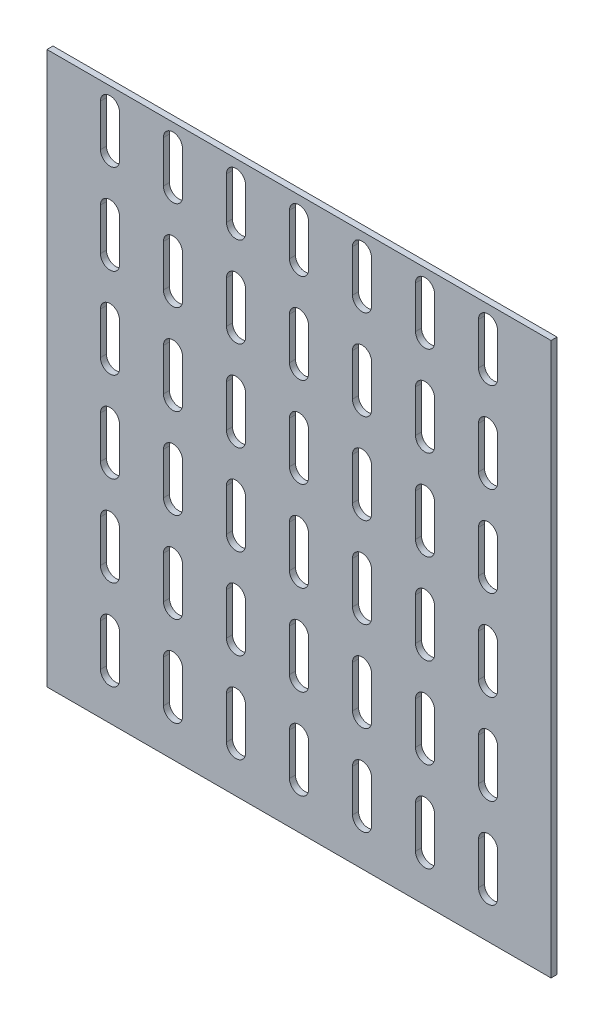
from build123d import *

# Parameters (mm, degrees)
SKETCH1_W           = 840
SKETCH1_H           = 920
BOSS_EXTRUDE1_DEPTH = 10
CUT_EXTRUDE1_DEPTH  = 10


with BuildPart() as part:
    # Sketch1 → Boss-Extrude1 (new body)
    with BuildSketch(Plane.XY):
        with Locations((368.938021937, -411.010102206)):
            Rectangle(SKETCH1_W, SKETCH1_H)
    extrude(amount=BOSS_EXTRUDE1_DEPTH)

    # Sketch2 → Cut-Extrude1 (cut)
    with BuildSketch(Plane.XY.offset(10)):
        with BuildLine():
            Line((69.818326735, -731.010102206), (69.818326735, -801.010102206))
            ThreePointArc((69.818326735, -801.010102206), (53.938021937, -816.890407004), (38.057717139, -801.010102206))
            Line((38.057717139, -801.010102206), (38.057717139, -731.010102206))
            ThreePointArc((38.057717139, -731.010102206), (53.938021937, -715.129797408), (69.818326735, -731.010102206))
        make_face()
        with BuildLine():
            Line((174.818326735, -731.010102206), (174.818326735, -801.010102206))
            ThreePointArc((174.818326735, -801.010102206), (158.938021937, -816.890407004), (143.057717139, -801.010102206))
            Line((143.057717139, -801.010102206), (143.057717139, -731.010102206))
            ThreePointArc((143.057717139, -731.010102206), (158.938021937, -715.129797408), (174.818326735, -731.010102206))
        make_face()
        with BuildLine():
            Line((69.818326735, 18.989897794), (69.818326735, -51.010102206))
            ThreePointArc((69.818326735, -51.010102206), (53.938021937, -66.890407004), (38.057717139, -51.010102206))
            Line((38.057717139, -51.010102206), (38.057717139, 18.989897794))
            ThreePointArc((38.057717139, 18.989897794), (53.938021937, 34.870202592), (69.818326735, 18.989897794))
        make_face()
        with BuildLine():
            Line((174.818326735, 18.989897794), (174.818326735, -51.010102206))
            ThreePointArc((174.818326735, -51.010102206), (158.938021937, -66.890407004), (143.057717139, -51.010102206))
            Line((143.057717139, -51.010102206), (143.057717139, 18.989897794))
            ThreePointArc((143.057717139, 18.989897794), (158.938021937, 34.870202592), (174.818326735, 18.989897794))
        make_face()
        with BuildLine():
            Line((279.818326735, 18.989897794), (279.818326735, -51.010102206))
            ThreePointArc((279.818326735, -51.010102206), (263.938021937, -66.890407004), (248.057717139, -51.010102206))
            Line((248.057717139, -51.010102206), (248.057717139, 18.989897794))
            ThreePointArc((248.057717139, 18.989897794), (263.938021937, 34.870202592), (279.818326735, 18.989897794))
        make_face()
        with BuildLine():
            Line((384.818326735, 18.989897794), (384.818326735, -51.010102206))
            ThreePointArc((384.818326735, -51.010102206), (368.938021937, -66.890407004), (353.057717139, -51.010102206))
            Line((353.057717139, -51.010102206), (353.057717139, 18.989897794))
            ThreePointArc((353.057717139, 18.989897794), (368.938021937, 34.870202592), (384.818326735, 18.989897794))
        make_face()
        with BuildLine():
            Line((489.818326735, 18.989897794), (489.818326735, -51.010102206))
            ThreePointArc((489.818326735, -51.010102206), (473.938021937, -66.890407004), (458.057717139, -51.010102206))
            Line((458.057717139, -51.010102206), (458.057717139, 18.989897794))
            ThreePointArc((458.057717139, 18.989897794), (473.938021937, 34.870202592), (489.818326735, 18.989897794))
        make_face()
        with BuildLine():
            Line((594.818326735, 18.989897794), (594.818326735, -51.010102206))
            ThreePointArc((594.818326735, -51.010102206), (578.938021937, -66.890407004), (563.057717139, -51.010102206))
            Line((563.057717139, -51.010102206), (563.057717139, 18.989897794))
            ThreePointArc((563.057717139, 18.989897794), (578.938021937, 34.870202592), (594.818326735, 18.989897794))
        make_face()
        with BuildLine():
            Line((699.818326735, 18.989897794), (699.818326735, -51.010102206))
            ThreePointArc((699.818326735, -51.010102206), (683.938021937, -66.890407004), (668.057717139, -51.010102206))
            Line((668.057717139, -51.010102206), (668.057717139, 18.989897794))
            ThreePointArc((668.057717139, 18.989897794), (683.938021937, 34.870202592), (699.818326735, 18.989897794))
        make_face()
        with BuildLine():
            Line((69.818326735, -131.010102206), (69.818326735, -201.010102206))
            ThreePointArc((69.818326735, -201.010102206), (53.938021937, -216.890407004), (38.057717139, -201.010102206))
            Line((38.057717139, -201.010102206), (38.057717139, -131.010102206))
            ThreePointArc((38.057717139, -131.010102206), (53.938021937, -115.129797408), (69.818326735, -131.010102206))
        make_face()
        with BuildLine():
            Line((174.818326735, -131.010102206), (174.818326735, -201.010102206))
            ThreePointArc((174.818326735, -201.010102206), (158.938021937, -216.890407004), (143.057717139, -201.010102206))
            Line((143.057717139, -201.010102206), (143.057717139, -131.010102206))
            ThreePointArc((143.057717139, -131.010102206), (158.938021937, -115.129797408), (174.818326735, -131.010102206))
        make_face()
        with BuildLine():
            Line((279.818326735, -131.010102206), (279.818326735, -201.010102206))
            ThreePointArc((279.818326735, -201.010102206), (263.938021937, -216.890407004), (248.057717139, -201.010102206))
            Line((248.057717139, -201.010102206), (248.057717139, -131.010102206))
            ThreePointArc((248.057717139, -131.010102206), (263.938021937, -115.129797408), (279.818326735, -131.010102206))
        make_face()
        with BuildLine():
            Line((384.818326735, -131.010102206), (384.818326735, -201.010102206))
            ThreePointArc((384.818326735, -201.010102206), (368.938021937, -216.890407004), (353.057717139, -201.010102206))
            Line((353.057717139, -201.010102206), (353.057717139, -131.010102206))
            ThreePointArc((353.057717139, -131.010102206), (368.938021937, -115.129797408), (384.818326735, -131.010102206))
        make_face()
        with BuildLine():
            Line((489.818326735, -131.010102206), (489.818326735, -201.010102206))
            ThreePointArc((489.818326735, -201.010102206), (473.938021937, -216.890407004), (458.057717139, -201.010102206))
            Line((458.057717139, -201.010102206), (458.057717139, -131.010102206))
            ThreePointArc((458.057717139, -131.010102206), (473.938021937, -115.129797408), (489.818326735, -131.010102206))
        make_face()
        with BuildLine():
            Line((594.818326735, -131.010102206), (594.818326735, -201.010102206))
            ThreePointArc((594.818326735, -201.010102206), (578.938021937, -216.890407004), (563.057717139, -201.010102206))
            Line((563.057717139, -201.010102206), (563.057717139, -131.010102206))
            ThreePointArc((563.057717139, -131.010102206), (578.938021937, -115.129797408), (594.818326735, -131.010102206))
        make_face()
        with BuildLine():
            Line((699.818326735, -131.010102206), (699.818326735, -201.010102206))
            ThreePointArc((699.818326735, -201.010102206), (683.938021937, -216.890407004), (668.057717139, -201.010102206))
            Line((668.057717139, -201.010102206), (668.057717139, -131.010102206))
            ThreePointArc((668.057717139, -131.010102206), (683.938021937, -115.129797408), (699.818326735, -131.010102206))
        make_face()
        with BuildLine():
            Line((69.818326735, -281.010102206), (69.818326735, -351.010102206))
            ThreePointArc((69.818326735, -351.010102206), (53.938021937, -366.890407004), (38.057717139, -351.010102206))
            Line((38.057717139, -351.010102206), (38.057717139, -281.010102206))
            ThreePointArc((38.057717139, -281.010102206), (53.938021937, -265.129797408), (69.818326735, -281.010102206))
        make_face()
        with BuildLine():
            Line((174.818326735, -281.010102206), (174.818326735, -351.010102206))
            ThreePointArc((174.818326735, -351.010102206), (158.938021937, -366.890407004), (143.057717139, -351.010102206))
            Line((143.057717139, -351.010102206), (143.057717139, -281.010102206))
            ThreePointArc((143.057717139, -281.010102206), (158.938021937, -265.129797408), (174.818326735, -281.010102206))
        make_face()
        with BuildLine():
            Line((279.818326735, -281.010102206), (279.818326735, -351.010102206))
            ThreePointArc((279.818326735, -351.010102206), (263.938021937, -366.890407004), (248.057717139, -351.010102206))
            Line((248.057717139, -351.010102206), (248.057717139, -281.010102206))
            ThreePointArc((248.057717139, -281.010102206), (263.938021937, -265.129797408), (279.818326735, -281.010102206))
        make_face()
        with BuildLine():
            Line((384.818326735, -281.010102206), (384.818326735, -351.010102206))
            ThreePointArc((384.818326735, -351.010102206), (368.938021937, -366.890407004), (353.057717139, -351.010102206))
            Line((353.057717139, -351.010102206), (353.057717139, -281.010102206))
            ThreePointArc((353.057717139, -281.010102206), (368.938021937, -265.129797408), (384.818326735, -281.010102206))
        make_face()
        with BuildLine():
            Line((489.818326735, -281.010102206), (489.818326735, -351.010102206))
            ThreePointArc((489.818326735, -351.010102206), (473.938021937, -366.890407004), (458.057717139, -351.010102206))
            Line((458.057717139, -351.010102206), (458.057717139, -281.010102206))
            ThreePointArc((458.057717139, -281.010102206), (473.938021937, -265.129797408), (489.818326735, -281.010102206))
        make_face()
        with BuildLine():
            Line((594.818326735, -281.010102206), (594.818326735, -351.010102206))
            ThreePointArc((594.818326735, -351.010102206), (578.938021937, -366.890407004), (563.057717139, -351.010102206))
            Line((563.057717139, -351.010102206), (563.057717139, -281.010102206))
            ThreePointArc((563.057717139, -281.010102206), (578.938021937, -265.129797408), (594.818326735, -281.010102206))
        make_face()
        with BuildLine():
            Line((699.818326735, -281.010102206), (699.818326735, -351.010102206))
            ThreePointArc((699.818326735, -351.010102206), (683.938021937, -366.890407004), (668.057717139, -351.010102206))
            Line((668.057717139, -351.010102206), (668.057717139, -281.010102206))
            ThreePointArc((668.057717139, -281.010102206), (683.938021937, -265.129797408), (699.818326735, -281.010102206))
        make_face()
        with BuildLine():
            Line((69.818326735, -431.010102206), (69.818326735, -501.010102206))
            ThreePointArc((69.818326735, -501.010102206), (53.938021937, -516.890407004), (38.057717139, -501.010102206))
            Line((38.057717139, -501.010102206), (38.057717139, -431.010102206))
            ThreePointArc((38.057717139, -431.010102206), (53.938021937, -415.129797408), (69.818326735, -431.010102206))
        make_face()
        with BuildLine():
            Line((174.818326735, -431.010102206), (174.818326735, -501.010102206))
            ThreePointArc((174.818326735, -501.010102206), (158.938021937, -516.890407004), (143.057717139, -501.010102206))
            Line((143.057717139, -501.010102206), (143.057717139, -431.010102206))
            ThreePointArc((143.057717139, -431.010102206), (158.938021937, -415.129797408), (174.818326735, -431.010102206))
        make_face()
        with BuildLine():
            Line((279.818326735, -431.010102206), (279.818326735, -501.010102206))
            ThreePointArc((279.818326735, -501.010102206), (263.938021937, -516.890407004), (248.057717139, -501.010102206))
            Line((248.057717139, -501.010102206), (248.057717139, -431.010102206))
            ThreePointArc((248.057717139, -431.010102206), (263.938021937, -415.129797408), (279.818326735, -431.010102206))
        make_face()
        with BuildLine():
            Line((384.818326735, -431.010102206), (384.818326735, -501.010102206))
            ThreePointArc((384.818326735, -501.010102206), (368.938021937, -516.890407004), (353.057717139, -501.010102206))
            Line((353.057717139, -501.010102206), (353.057717139, -431.010102206))
            ThreePointArc((353.057717139, -431.010102206), (368.938021937, -415.129797408), (384.818326735, -431.010102206))
        make_face()
        with BuildLine():
            Line((489.818326735, -431.010102206), (489.818326735, -501.010102206))
            ThreePointArc((489.818326735, -501.010102206), (473.938021937, -516.890407004), (458.057717139, -501.010102206))
            Line((458.057717139, -501.010102206), (458.057717139, -431.010102206))
            ThreePointArc((458.057717139, -431.010102206), (473.938021937, -415.129797408), (489.818326735, -431.010102206))
        make_face()
        with BuildLine():
            Line((594.818326735, -431.010102206), (594.818326735, -501.010102206))
            ThreePointArc((594.818326735, -501.010102206), (578.938021937, -516.890407004), (563.057717139, -501.010102206))
            Line((563.057717139, -501.010102206), (563.057717139, -431.010102206))
            ThreePointArc((563.057717139, -431.010102206), (578.938021937, -415.129797408), (594.818326735, -431.010102206))
        make_face()
        with BuildLine():
            Line((699.818326735, -431.010102206), (699.818326735, -501.010102206))
            ThreePointArc((699.818326735, -501.010102206), (683.938021937, -516.890407004), (668.057717139, -501.010102206))
            Line((668.057717139, -501.010102206), (668.057717139, -431.010102206))
            ThreePointArc((668.057717139, -431.010102206), (683.938021937, -415.129797408), (699.818326735, -431.010102206))
        make_face()
        with BuildLine():
            Line((69.818326735, -581.010102206), (69.818326735, -651.010102206))
            ThreePointArc((69.818326735, -651.010102206), (53.938021937, -666.890407004), (38.057717139, -651.010102206))
            Line((38.057717139, -651.010102206), (38.057717139, -581.010102206))
            ThreePointArc((38.057717139, -581.010102206), (53.938021937, -565.129797408), (69.818326735, -581.010102206))
        make_face()
        with BuildLine():
            Line((174.818326735, -581.010102206), (174.818326735, -651.010102206))
            ThreePointArc((174.818326735, -651.010102206), (158.938021937, -666.890407004), (143.057717139, -651.010102206))
            Line((143.057717139, -651.010102206), (143.057717139, -581.010102206))
            ThreePointArc((143.057717139, -581.010102206), (158.938021937, -565.129797408), (174.818326735, -581.010102206))
        make_face()
        with BuildLine():
            Line((279.818326735, -581.010102206), (279.818326735, -651.010102206))
            ThreePointArc((279.818326735, -651.010102206), (263.938021937, -666.890407004), (248.057717139, -651.010102206))
            Line((248.057717139, -651.010102206), (248.057717139, -581.010102206))
            ThreePointArc((248.057717139, -581.010102206), (263.938021937, -565.129797408), (279.818326735, -581.010102206))
        make_face()
        with BuildLine():
            Line((384.818326735, -581.010102206), (384.818326735, -651.010102206))
            ThreePointArc((384.818326735, -651.010102206), (368.938021937, -666.890407004), (353.057717139, -651.010102206))
            Line((353.057717139, -651.010102206), (353.057717139, -581.010102206))
            ThreePointArc((353.057717139, -581.010102206), (368.938021937, -565.129797408), (384.818326735, -581.010102206))
        make_face()
        with BuildLine():
            Line((489.818326735, -581.010102206), (489.818326735, -651.010102206))
            ThreePointArc((489.818326735, -651.010102206), (473.938021937, -666.890407004), (458.057717139, -651.010102206))
            Line((458.057717139, -651.010102206), (458.057717139, -581.010102206))
            ThreePointArc((458.057717139, -581.010102206), (473.938021937, -565.129797408), (489.818326735, -581.010102206))
        make_face()
        with BuildLine():
            Line((594.818326735, -581.010102206), (594.818326735, -651.010102206))
            ThreePointArc((594.818326735, -651.010102206), (578.938021937, -666.890407004), (563.057717139, -651.010102206))
            Line((563.057717139, -651.010102206), (563.057717139, -581.010102206))
            ThreePointArc((563.057717139, -581.010102206), (578.938021937, -565.129797408), (594.818326735, -581.010102206))
        make_face()
        with BuildLine():
            Line((699.818326735, -581.010102206), (699.818326735, -651.010102206))
            ThreePointArc((699.818326735, -651.010102206), (683.938021937, -666.890407004), (668.057717139, -651.010102206))
            Line((668.057717139, -651.010102206), (668.057717139, -581.010102206))
            ThreePointArc((668.057717139, -581.010102206), (683.938021937, -565.129797408), (699.818326735, -581.010102206))
        make_face()
        with BuildLine():
            Line((279.818326735, -731.010102206), (279.818326735, -801.010102206))
            ThreePointArc((279.818326735, -801.010102206), (263.938021937, -816.890407004), (248.057717139, -801.010102206))
            Line((248.057717139, -801.010102206), (248.057717139, -731.010102206))
            ThreePointArc((248.057717139, -731.010102206), (263.938021937, -715.129797408), (279.818326735, -731.010102206))
        make_face()
        with BuildLine():
            Line((384.818326735, -731.010102206), (384.818326735, -801.010102206))
            ThreePointArc((384.818326735, -801.010102206), (368.938021937, -816.890407004), (353.057717139, -801.010102206))
            Line((353.057717139, -801.010102206), (353.057717139, -731.010102206))
            ThreePointArc((353.057717139, -731.010102206), (368.938021937, -715.129797408), (384.818326735, -731.010102206))
        make_face()
        with BuildLine():
            Line((489.818326735, -731.010102206), (489.818326735, -801.010102206))
            ThreePointArc((489.818326735, -801.010102206), (473.938021937, -816.890407004), (458.057717139, -801.010102206))
            Line((458.057717139, -801.010102206), (458.057717139, -731.010102206))
            ThreePointArc((458.057717139, -731.010102206), (473.938021937, -715.129797408), (489.818326735, -731.010102206))
        make_face()
        with BuildLine():
            Line((594.818326735, -731.010102206), (594.818326735, -801.010102206))
            ThreePointArc((594.818326735, -801.010102206), (578.938021937, -816.890407004), (563.057717139, -801.010102206))
            Line((563.057717139, -801.010102206), (563.057717139, -731.010102206))
            ThreePointArc((563.057717139, -731.010102206), (578.938021937, -715.129797408), (594.818326735, -731.010102206))
        make_face()
        with BuildLine():
            Line((699.818326735, -731.010102206), (699.818326735, -801.010102206))
            ThreePointArc((699.818326735, -801.010102206), (683.938021937, -816.890407004), (668.057717139, -801.010102206))
            Line((668.057717139, -801.010102206), (668.057717139, -731.010102206))
            ThreePointArc((668.057717139, -731.010102206), (683.938021937, -715.129797408), (699.818326735, -731.010102206))
        make_face()
    extrude(amount=-CUT_EXTRUDE1_DEPTH, mode=Mode.SUBTRACT)


solid = part.part
